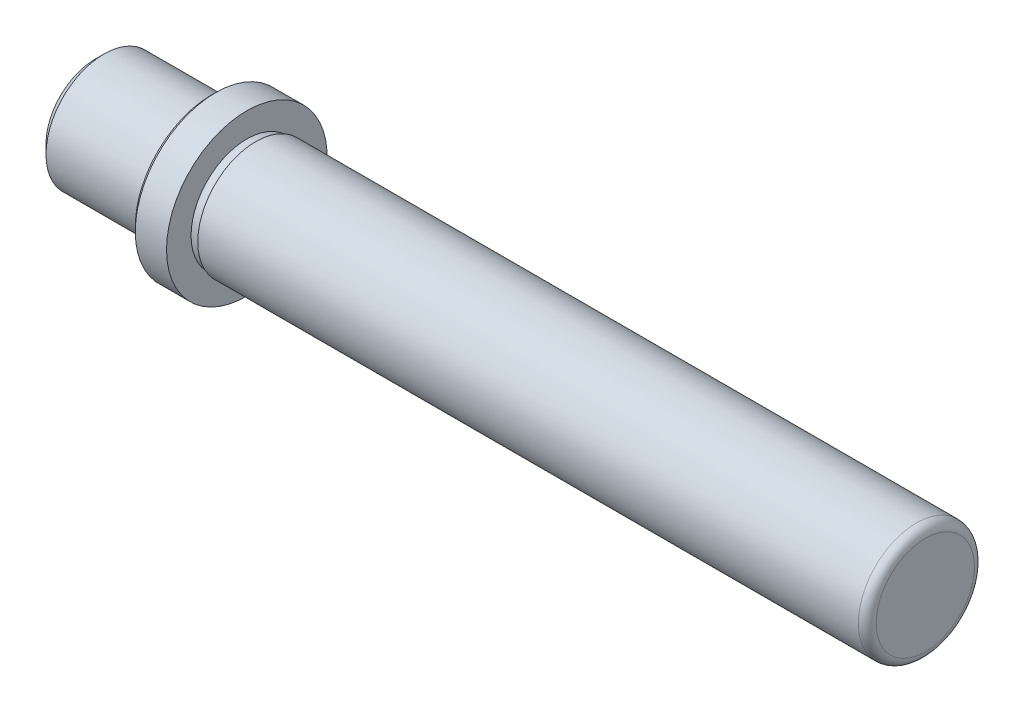
SolidWorks part; units mm, degrees
ref_plane "Front Plane" through (0, 0, 0) normal (0, 0, 1) x (1, 0, 0)
ref_plane "Top Plane" through (0, 0, 0) normal (0, 1, 0) x (1, 0, 0)
ref_plane "Right Plane" through (0, 0, 0) normal (1, 0, 0) x (0, 0, -1)
sketch "Sketch1" plane through (0, 0, 0) normal (0, 0, 1) x (1, 0, 0)
  line L0 (0, 0) -> (128.5196, 0) construction
  line L1 (13, 6.5) -> (13, 9)
  line L2 (13, 9) -> (17, 9)
  line L3 (17, 9) -> (17, 6.25)
  line L4 (17, 6.25) -> (18, 6.25)
  line L5 (18, 6.25) -> (18, 6.5)
  line L6 (18, 6.5) -> (93, 6.5)
  line L7 (93, 6.5) -> (93, 0)
  line L8 (0, 0) -> (93, 0)
  line L9 (13, 6.5) -> (0, 6.5)
  line L10 (0, 6.5) -> (0, 0)
  dimension "D1" = 18
  dimension "D2" = 4
  dimension "D3" = 1
  dimension "D4" = 12.5
  dimension "D5" = 13
  dimension "D6" = 80
  dimension "D7" = 13
revolve "Revolve1" add sketch "Sketch1" angle 360 about L0
fillet "Fillet1" radius 1 1 edges at (93, 0, 6.5)
chamfer "Chamfer1" distance 0.5 angle 45 1 edges at (13, 0, 9)
chamfer "Chamfer2" distance 1 angle 45 1 edges at (0, 0, 6.5)
hole_wizard "M5 Tapped Hole1" positions "Sketch3" profile "Sketch2" tap size "M5" standard "GB"
sketch "Sketch3" plane through (0, 0, 0) normal (-1, 0, 0) x (0, 0, 1)
  point P0 (0, 0)
sketch "Sketch2" plane through (0, 0, 0) normal (0, 1, 0) x (0, 0, 1)
  line L0 (0, 0) -> (0, 15.2618)
  line L1 (0, 15.2618) -> (2.1, 14)
  line L2 (2.1, 14) -> (2.1, 0)
  line L5 (2.1, 0) -> (0, 0)
  line L10 (0, 15.2618) -> (-2.1, 14) construction
  line L11 (0, -6.35) -> (0, 107.95) construction
  dimension "螺纹孔钻头直径" = 4.2
  dimension "螺纹孔钻头深度" = 14
  dimension "导头角度" = 118
cosmetic thread "Hole cosmetic thread1" parameters "D1"=10, "D2"=5
